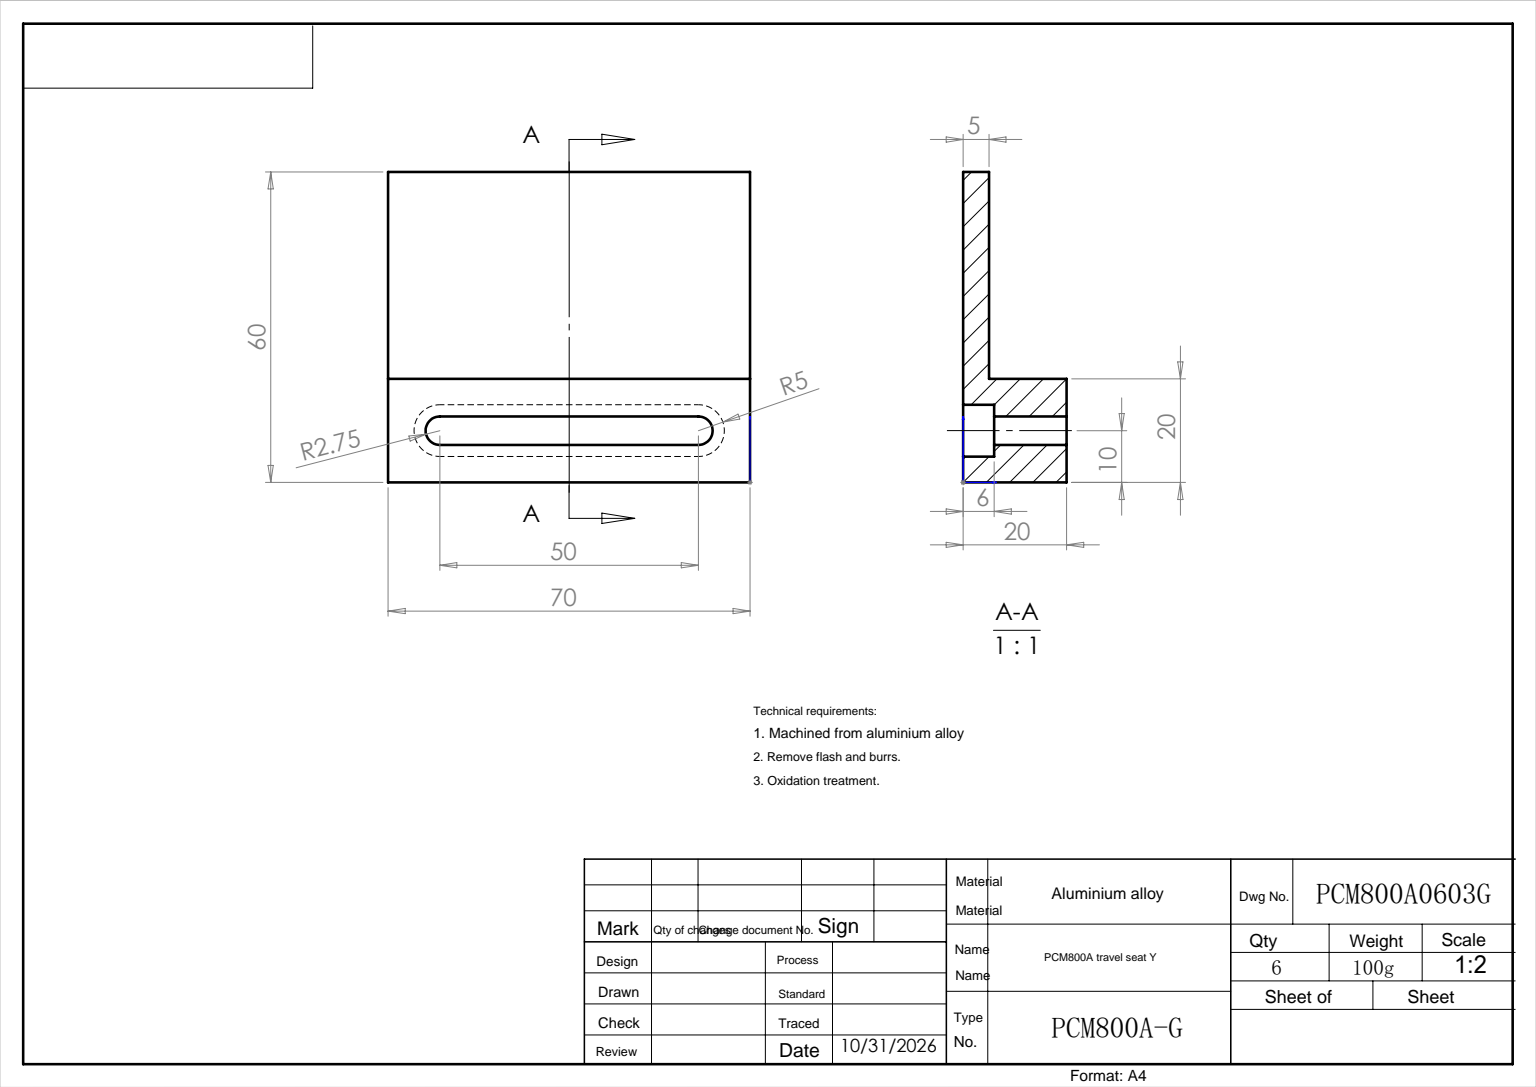
from build123d import *

# Parameters (mm, degrees)
EXTRUDE_1_DEPTH     = 70
CUT_EXTRUDE_1_DEPTH = 1200
CUT_EXTRUDE_2_DEPTH = 6


with BuildPart() as part:
    # 草图1 → 凸台-拉伸1 (new body)
    with BuildSketch(Plane.XY):
        Polygon((0, 0), (0, 60), (5, 60), (5, 20), (20, 20), (20, 0), align=None)
    extrude(amount=EXTRUDE_1_DEPTH)

    # 草图3 → 切除-拉伸1 (cut)
    with BuildSketch(Plane.ZY):
        with BuildLine():
            Line((10, 12.75), (60, 12.75))
            ThreePointArc((60, 12.75), (62.75, 10), (60, 7.25))
            Line((60, 7.25), (10, 7.25))
            ThreePointArc((10, 7.25), (7.25, 10), (10, 12.75))
        make_face()
    extrude(amount=-CUT_EXTRUDE_1_DEPTH, mode=Mode.SUBTRACT)

    # 草图6 → 切除-拉伸2 (cut)
    with BuildSketch(Plane.ZY):
        with BuildLine():
            Line((10, 5), (60, 5))
            ThreePointArc((60, 5), (65, 10), (60, 15))
            Line((60, 15), (10, 15))
            ThreePointArc((10, 15), (5, 10), (10, 5))
        make_face()
    extrude(amount=-CUT_EXTRUDE_2_DEPTH, mode=Mode.SUBTRACT)


solid = part.part
